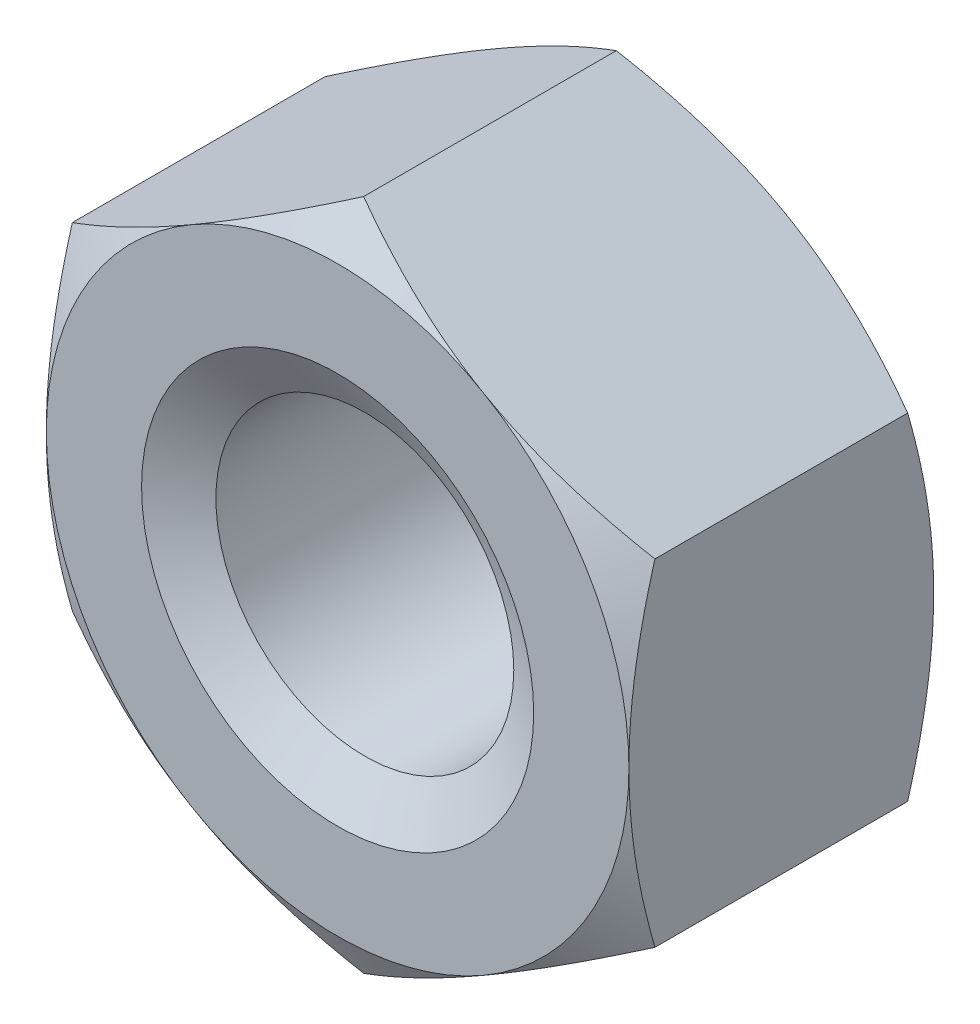
from build123d import *

# Parameters (mm, degrees)
SKETCH_3_R          = 3.3234375
EXTRUDE_1_DEPTH     = 6.8
SKETCH_5_R          = 10.785
SKETCH_5_R_2        = 6.5
CUT_EXTRUDE_1_DEPTH = 1.36
CUT_EXTRUDE_1_DRAFT = -60
SKETCH_7_R          = 10.785
SKETCH_7_R_2        = 6.5
CUT_EXTRUDE_2_DEPTH = 1.36
CUT_EXTRUDE_2_DRAFT = -60


with BuildPart() as part:
    # 草图3 → 凸台-拉伸1 (new body)
    with BuildSketch(Plane.XY):
        Polygon((0, 7.505553499), (-6.5, 3.75277675), (-6.5, -3.75277675), (0, -7.505553499), (6.5, -3.75277675), (6.5, 3.75277675), align=None)
        Circle(SKETCH_3_R, mode=Mode.SUBTRACT)
    extrude(amount=-EXTRUDE_1_DEPTH)

    # 草图4 → 切除-旋转1 (revolve, cut)
    with BuildSketch(Plane(origin=(0, 0, 0), x_dir=(0, 0, -1), z_dir=(1, 0, 0)), mode=Mode.PRIVATE) as cut_revolve_1_sk:
        Polygon((0, 4.375), (0.607119892, 3.3234375), (0.607119892, 0), (0, 0), align=None)
        Polygon((6.8, 0), (6.8, 4.375), (6.192880108, 3.3234375), (6.192880108, 0), align=None)
    revolve(cut_revolve_1_sk.sketch.rotate(Axis((0, 0, 0), (0, 0, -1)), 90), axis=Axis((0, 0, 0), (0, 0, -1)), mode=Mode.SUBTRACT)


with BuildPart() as cut_extrude_1_tool:
    # 草图5 → 切除-拉伸1 (with draft: the straight prism first)
    with BuildSketch(Plane.XY):
        Circle(SKETCH_5_R)
        Circle(SKETCH_5_R_2, mode=Mode.SUBTRACT)
    extrude(amount=-CUT_EXTRUDE_1_DEPTH)
    # 切除-拉伸1: the draft: its side faces are tilted about the plane it starts from
    cut_extrude_1_sides = [cut_extrude_1_tool.faces().sort_by_distance(p)[0] for p in [
        (-10.785, 0, -0.68),
        (-6.5, 0, -0.68),
    ]]
    draft(cut_extrude_1_sides, Plane.XY, CUT_EXTRUDE_1_DRAFT)


with BuildPart() as part_1:
    add(part.part)

    # 切除-拉伸1: cut by cut_extrude_1_tool
    add(cut_extrude_1_tool.part, mode=Mode.SUBTRACT)


with BuildPart() as cut_extrude_2_tool:
    # 草图7 → 切除-拉伸2 (with draft: the straight prism first)
    with BuildSketch(Plane(origin=(0, 0, -6.8), x_dir=(-1, 0, 0), z_dir=(0, 0, -1))):
        Circle(SKETCH_7_R)
        Circle(SKETCH_7_R_2, mode=Mode.SUBTRACT)
    extrude(amount=-CUT_EXTRUDE_2_DEPTH)
    # 切除-拉伸2: the draft: its side faces are tilted about the plane it starts from
    cut_extrude_2_sides = [cut_extrude_2_tool.faces().sort_by_distance(p)[0] for p in [
        (10.785, 0, -6.12),
        (6.5, 0, -6.12),
    ]]
    draft(cut_extrude_2_sides, Plane(origin=(0, 0, -6.8), x_dir=(-1, 0, 0), z_dir=(0, 0, -1)), CUT_EXTRUDE_2_DRAFT)


with BuildPart() as part_2:
    add(part_1.part)

    # 切除-拉伸2: cut by cut_extrude_2_tool
    add(cut_extrude_2_tool.part, mode=Mode.SUBTRACT)


solid = part_2.part
